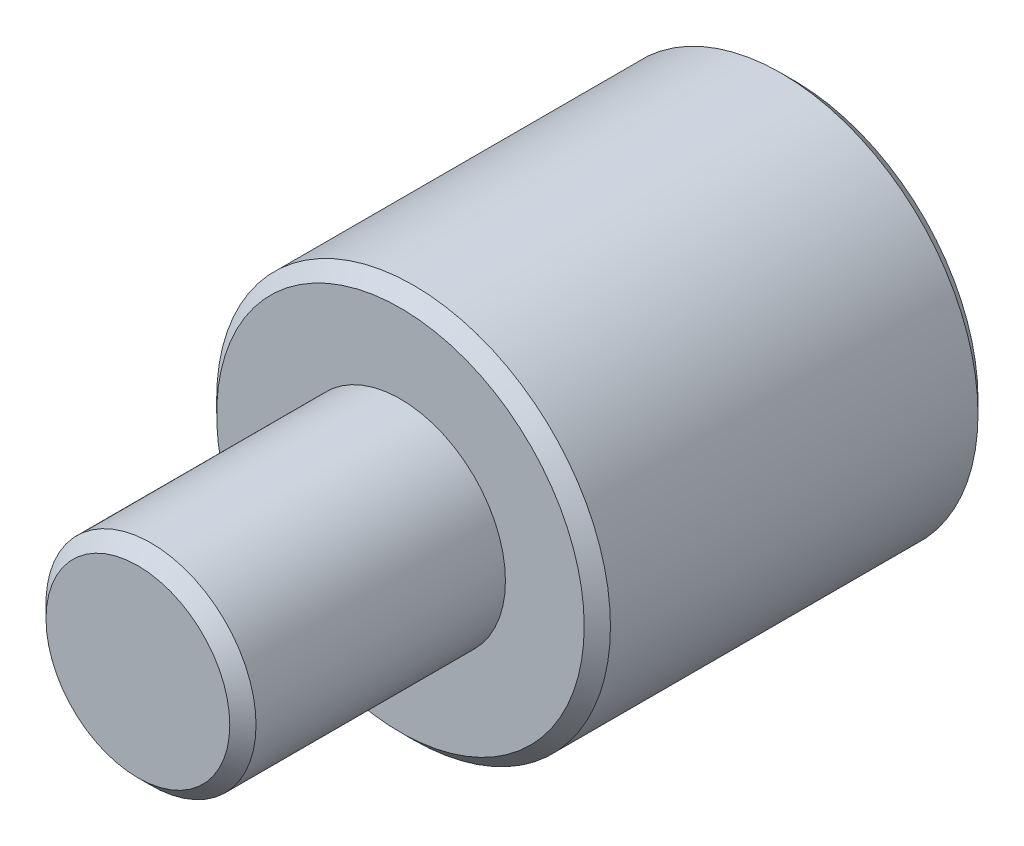
SolidWorks part; units mm, degrees
ref_plane "Front Plane" through (0, 0, 0) normal (0, 0, 1) x (1, 0, 0)
ref_plane "Top Plane" through (0, 0, 0) normal (0, 1, 0) x (1, 0, 0)
ref_plane "Right Plane" through (0, 0, 0) normal (1, 0, 0) x (0, 0, -1)
sketch "Sketch1" plane through (0, 0, 0) normal (0, 0, 1) x (1, 0, 0)
  circle A0 centre (0, 0) radius 7.5
  dimension "D1" = 15
extrude "Boss-Extrude1" add sketch "Sketch1" along normal blind 15
sketch "Sketch2" plane through (0, 0, 15) normal (0, 0, 1) x (1, 0, 0)
  circle A0 centre (0, 0) radius 4
  dimension "D1" = 8
extrude "Boss-Extrude2" add sketch "Sketch2" along normal blind 10
chamfer "Chamfer1" distance 0.5 angle 45 3 edges at (7.5, 0, 0) (7.5, 0, 15) (4, 0, 25)
